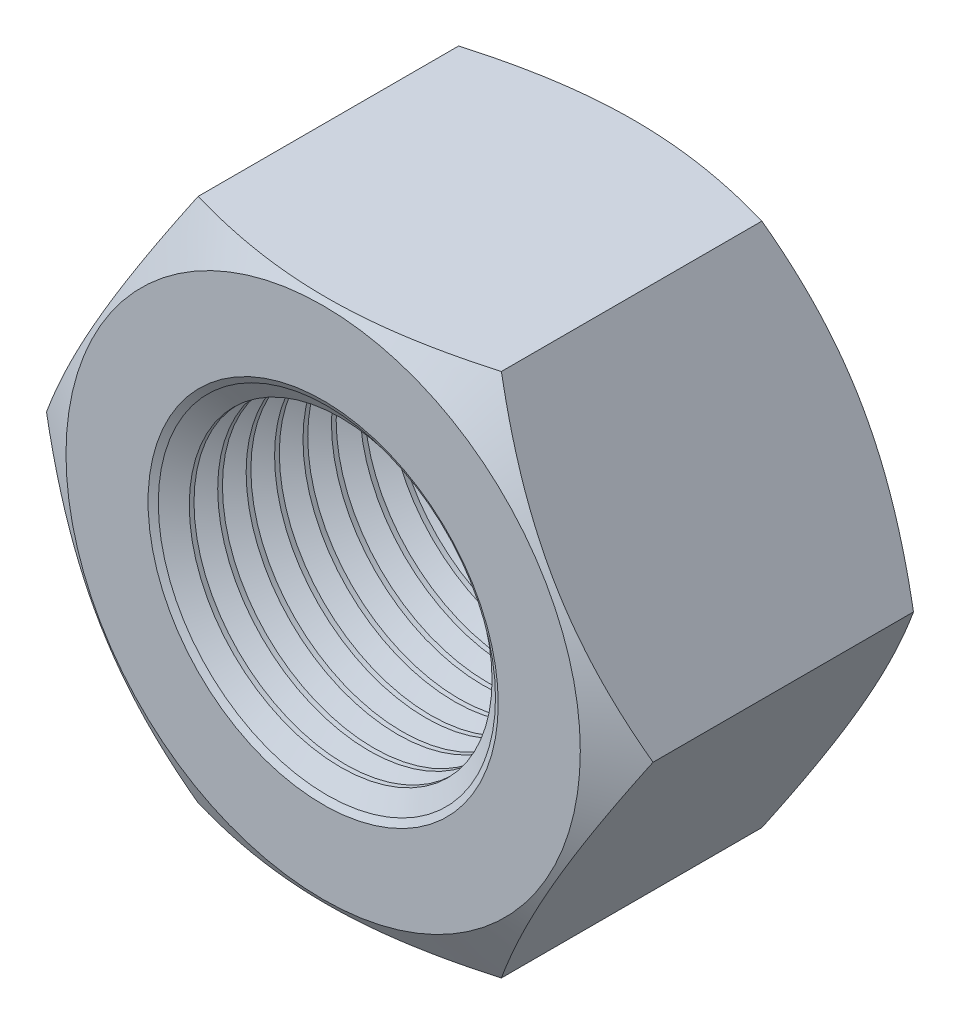
SolidWorks part; units mm, degrees
ref_plane "Front" through (0, 0, 0) normal (0, 0, 1) x (1, 0, 0)
ref_plane "Top" through (0, 0, 0) normal (0, 1, 0) x (1, 0, 0)
ref_plane "Right" through (0, 0, 0) normal (1, 0, 0) x (0, 0, -1)
sketch "Sketch1" plane through (0, 0, 0) normal (0, 0, 1) x (1, 0, 0)
  line L1 (20.7846, 0) -> (10.3923, 18)
  line L2 (10.3923, 18) -> (-10.3923, 18)
  line L3 (-10.3923, 18) -> (-20.7846, 0)
  line L4 (-20.7846, 0) -> (-10.3923, -18)
  line L5 (-10.3923, -18) -> (10.3923, -18)
  line L6 (10.3923, -18) -> (20.7846, 0)
  circle A0 centre (0, 0) radius 18 construction
  circle A1 centre (0, 0) radius 10.376
extrude "BaseNut" add sketch "Sketch1" against normal blind 21.5
cosmetic thread "ThreadCosmetic1" [suppressed] parameters "D"=24
sketch "Sketch2" plane through (0, 0, 0) normal (0, 1, 0) x (1, 0, 0)
  line L0 (-20.7846, 21.5) -> (-17.625, 21.5)
  line L2 (-17.625, 21.5) -> (-20.7846, 19.6758)
  line L3 (-20.7846, 19.6758) -> (-20.7846, 21.5)
  line L4 (0, 3.3759) -> (0, -9.8171) construction
  line L6 (-9.7712, 10.75) -> (9.8853, 10.75) construction
  line L7 (-20.7846, 1.8242) -> (-20.7846, 0)
  line L8 (-17.625, 0) -> (-20.7846, 1.8242)
  line L9 (-20.7846, 0) -> (-17.625, 0)
revolve "Double-Chamfer" cut sketch "Sketch2" angle 360 about L4
chamfer "EndChamfer" distance 1.624 angle 30 2 edges at (10.376, 0, -21.5) (10.376, 0, 0)
sketch "Sketch3" plane through (0, 0, 0) normal (0, 1, 0) x (1, 0, 0)
  line L0 (-11.7824, 19.876) -> (-10.376, 19.064)
  line L1 (-10.376, 19.064) -> (-8.752, 19.064)
  line L2 (-8.752, 19.064) -> (-8.752, 20.688)
  line L3 (-8.752, 20.688) -> (-10.376, 20.688)
  line L4 (-10.376, 20.688) -> (-11.7824, 19.876)
  line L5 (0, 7.4383) -> (0, 16.8806) construction
revolve "Cut-Revolve10" cut sketch "Sketch3" angle 360 about L5
pattern_linear "LPattern10" count 11 spacing 1.9488 along (0, 0, 1) of "Cut-Revolve10"
equation "\"dw@Sketch2\" = \"s@Sketch1\"-0.75"
equation "\"D2@Sketch2\" = \"m@BaseNut\" / 2"
equation "\"D2@Sketch3\" = \"D@Sketch1\""
equation "\"D1@Sketch3\" =  (\"D@ThreadCosmetic1\"   - \"D@Sketch1\")  / 2"
equation "\"D3@LPattern10\" = \"D1@Sketch3\" * 1.2"
equation "\"D1@LPattern10\" = \"m@BaseNut\"/\"D3@LPattern10\""
